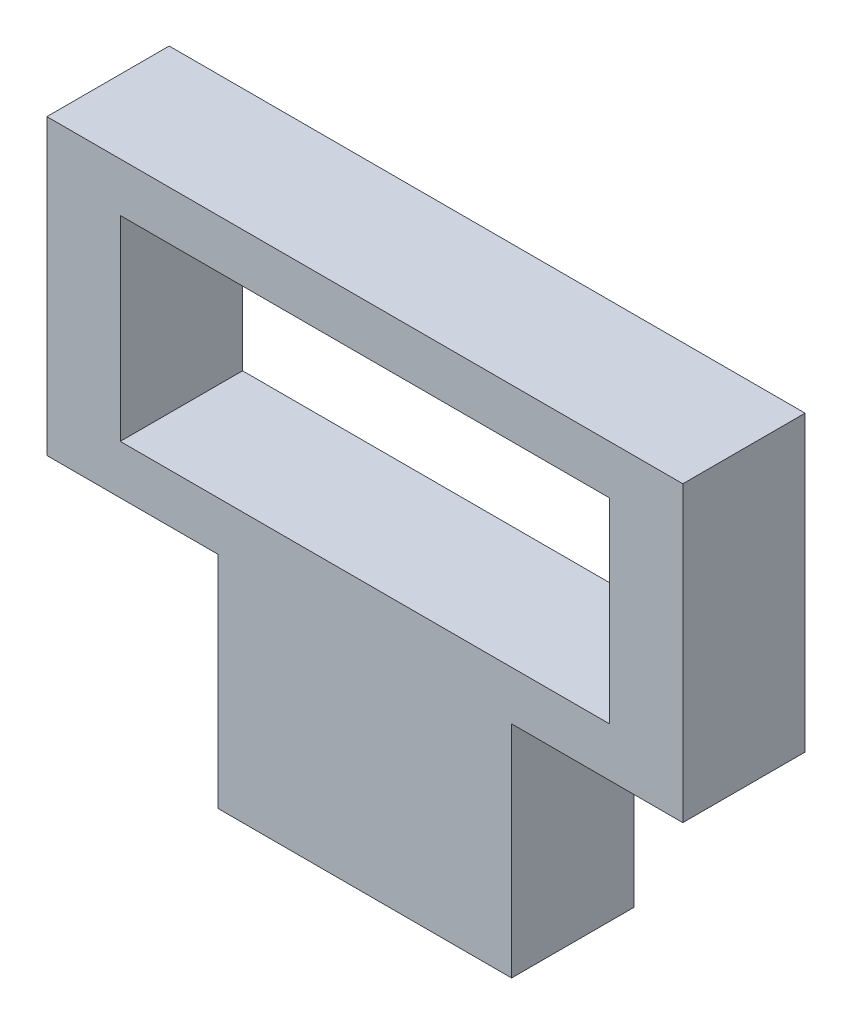
SolidWorks part; units mm, degrees
ref_plane "前视基准面" through (0, 0, 0) normal (0, 0, 1) x (1, 0, 0)
ref_plane "上视基准面" through (0, 0, 0) normal (0, 1, 0) x (1, 0, 0)
ref_plane "右视基准面" through (0, 0, 0) normal (1, 0, 0) x (0, 0, -1)
other "Configuration Table"
sketch "草图1" plane through (0, 0, 0) normal (0, 0, 1) x (1, 0, 0)
  line L0 (-13, -6) -> (13, -6)
  line L1 (13, -6) -> (13, 6)
  line L2 (13, 6) -> (-13, 6)
  line L3 (-13, 6) -> (-13, -6)
  line L4 (-10, -4) -> (10, -4)
  line L5 (10, -4) -> (10, 4)
  line L6 (10, 4) -> (-10, 4)
  line L7 (-10, 4) -> (-10, -4)
  point P0 (0, 0)
  dimension "D1" = 3
  dimension "D2" = 13
  dimension "D3" = 23
  dimension "D4" = 26
  dimension "D5" = 2
  dimension "D6" = 6
  dimension "D7" = 10
  dimension "D8" = 12
extrude "凸台-拉伸1" add sketch "草图1" against normal mid plane 5
sketch "草图2" plane through (0, 0, 0) normal (0, 0, 1) x (1, 0, 0)
  line L0 (-6, -15) -> (6, -15)
  line L1 (6, -15) -> (6, -6)
  line L2 (6, -6) -> (-6, -6)
  line L3 (-6, -6) -> (-6, -15)
  point P0 (0, 0)
  dimension "D1" = 6
  dimension "D2" = 12
  dimension "D3" = 9
  dimension "D4" = 15
extrude "凸台-拉伸2" add sketch "草图2" against normal mid plane 5
